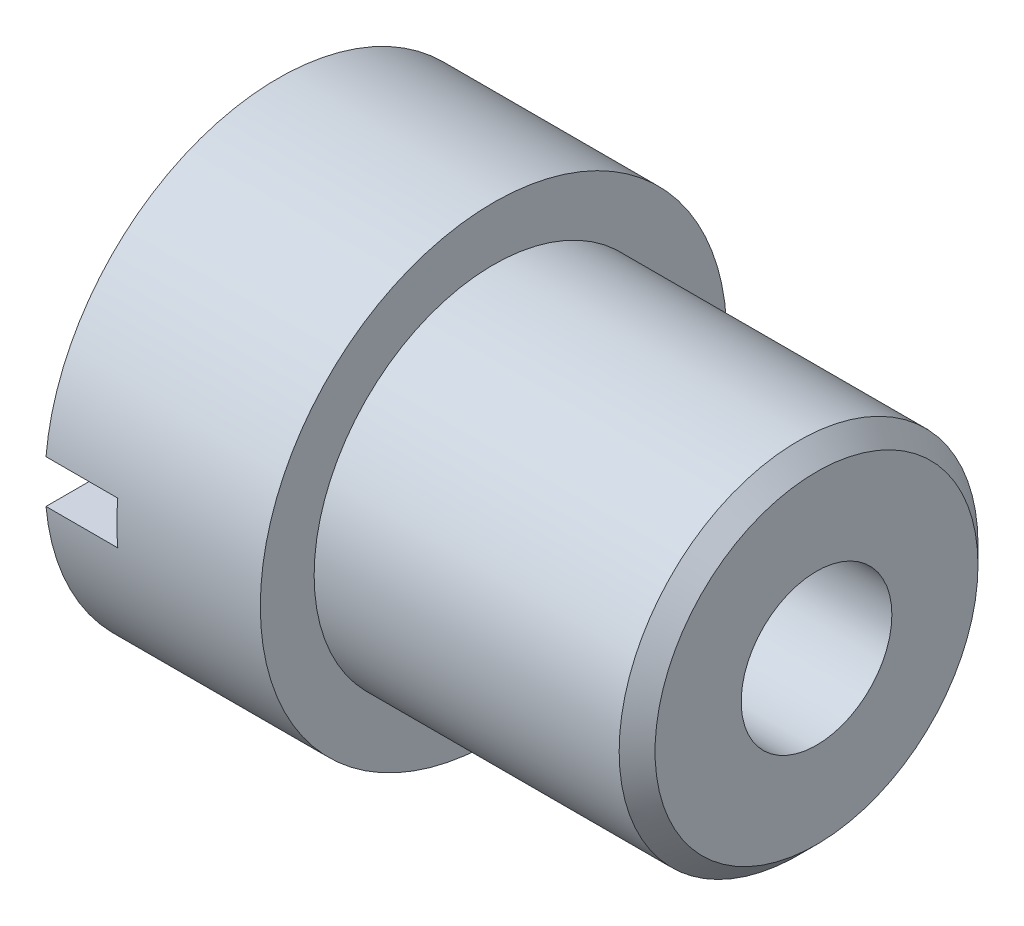
from build123d import *

# Parameters (mm, degrees)
SKETCH_2_R             = 5
EXTRUDE_1_DEPTH        = 9
SKETCH_5_R             = 6.5
EXTRUDE_2_DEPTH        = 6
SKETCH_6_W             = 30
SKETCH_6_H             = 1.2
CUT_EXTRUDE_1_DEPTH    = 2
HOLE_WIZARD_M5_1_D     = 4.2
HOLE_WIZARD_M5_1_DEPTH = 11
HOLE_WIZARD_M5_1_TIP   = 1.2618073
CHAMFER_1_SIZE         = 0.5


with BuildPart() as part:
    # 草图2 → 凸台-拉伸1 (new body)
    with BuildSketch(Plane(origin=(0, 0, 0), x_dir=(0, 0, -1), z_dir=(1, 0, 0))):
        Circle(SKETCH_2_R)
    extrude(amount=EXTRUDE_1_DEPTH)

    # 草图5 → 凸台-拉伸2 (add)
    with BuildSketch(Plane.ZY):
        Circle(SKETCH_5_R)
    extrude(amount=EXTRUDE_2_DEPTH)

    # 草图6 → 切除-拉伸1 (cut)
    with BuildSketch(Plane.ZY.offset(6)):
        Rectangle(SKETCH_6_W, SKETCH_6_H)
    extrude(amount=-CUT_EXTRUDE_1_DEPTH, mode=Mode.SUBTRACT)

    # M5 螺纹孔1
    with Locations(Plane(origin=(9, 0, 0), x_dir=(0, 0, 1), z_dir=(1, 0, 0))):
        with Locations((0, 0)):
            Hole(HOLE_WIZARD_M5_1_D / 2, depth=HOLE_WIZARD_M5_1_DEPTH)
            with Locations((0, 0, -(HOLE_WIZARD_M5_1_DEPTH + HOLE_WIZARD_M5_1_TIP / 2))):  # 118° drill point
                Cone(0, HOLE_WIZARD_M5_1_D / 2, HOLE_WIZARD_M5_1_TIP, mode=Mode.SUBTRACT)

    # 倒角1
    chamfer_1_edges = [part.edges().sort_by_distance(p)[0] for p in [
        (9, 0, 5),
    ]]
    chamfer(chamfer_1_edges, length=CHAMFER_1_SIZE)


solid = part.part
